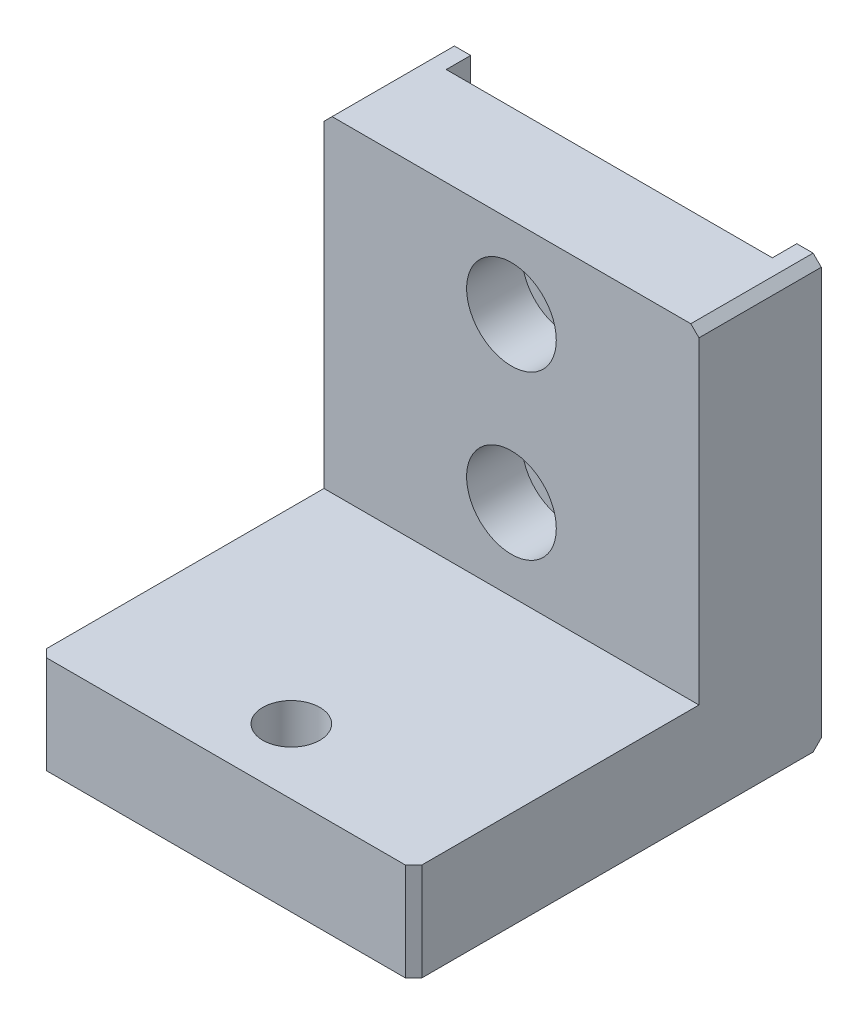
from build123d import *

# Parameters (mm, degrees)
SKETCH_1_W                = 46
SKETCH_1_H                = 50
EXTRUDE_1_DEPTH           = 6
SKETCH_2_W                = 46
SKETCH_2_H                = 15
EXTRUDE_2_DEPTH           = 40
SKETCH_3_W                = 40
SKETCH_3_H                = 52
CUT_EXTRUDE_1_DEPTH       = 3
CHAMFER_1_SIZE            = 1
HOLE_WIZARD_1_D           = 6.6
HOLE_WIZARD_1_CBORE_D     = 11
HOLE_WIZARD_1_CBORE_DEPTH = 6.8
M8X1_0_1_D                = 7


with BuildPart() as part:
    # 草图1 → 凸台-拉伸1 (new, symmetric)
    with BuildSketch(Plane(origin=(0, 0, 0), x_dir=(1, 0, 0), z_dir=(0, 1, 0))):
        Rectangle(SKETCH_1_W, SKETCH_1_H)
    extrude(amount=EXTRUDE_1_DEPTH, both=True)

    # 草图2 → 凸台-拉伸2 (add)
    with BuildSketch(Plane(origin=(0, 6, 0), x_dir=(1, 0, 0), z_dir=(0, 1, 0))):
        with Locations((0, 17.5)):
            Rectangle(SKETCH_2_W, SKETCH_2_H)
    extrude(amount=EXTRUDE_2_DEPTH)

    # 草图3 → 切除-拉伸1 (cut)
    with BuildSketch(Plane(origin=(0, 0, -25), x_dir=(-1, 0, 0), z_dir=(0, 0, -1))):
        with Locations((0, 20)):
            Rectangle(SKETCH_3_W, SKETCH_3_H)
    extrude(amount=-CUT_EXTRUDE_1_DEPTH, mode=Mode.SUBTRACT)

    # 倒角1
    chamfer_1_edges = [part.edges().sort_by_distance(p)[0] for p in [
        (23, 46, -17.5),
        (-23, 46, -17.5),
        (-21.5, -6, -25),
        (21.5, -6, -25),
        (23, 0, 25),
        (-23, 0, 25),
    ]]
    chamfer(chamfer_1_edges, length=CHAMFER_1_SIZE)

    # 打孔尺寸(%根据)内六角圆柱头螺钉的类型1 (through all)
    with Locations(Plane.XY.offset(-10)):
        with Locations((0, 16), (0, 36)):
            CounterBoreHole(HOLE_WIZARD_1_D / 2, HOLE_WIZARD_1_CBORE_D / 2, HOLE_WIZARD_1_CBORE_DEPTH)

    # M8x1.0 螺纹孔1 (through all)
    with Locations(Plane(origin=(0, 6, 0), x_dir=(1, 0, 0), z_dir=(0, 1, 0))):
        with Locations((0, -17)):
            Hole(M8X1_0_1_D / 2)


solid = part.part
